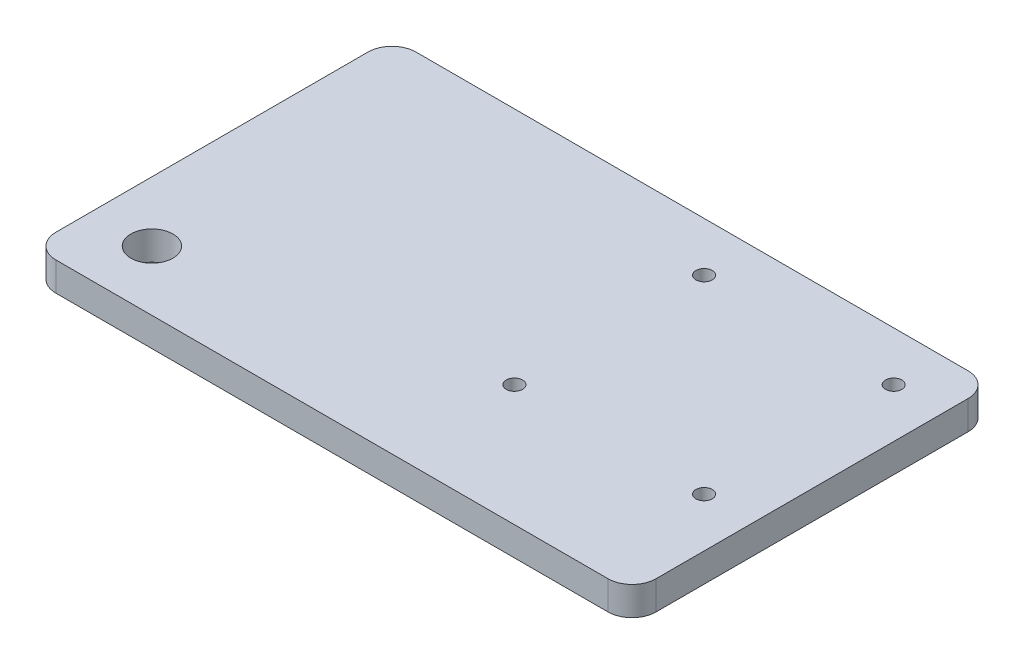
SolidWorks part; units mm, degrees
material "A3钢"
ref_plane "前视基准面" through (0, 0, 0) normal (0, 0, 1) x (1, 0, 0)
ref_plane "上视基准面" through (0, 0, 0) normal (0, 1, 0) x (1, 0, 0)
ref_plane "右视基准面" through (0, 0, 0) normal (1, 0, 0) x (0, 0, -1)
sketch "草图1" plane through (0, 0, 0) normal (0, 1, 0) x (1, 0, 0)
  line L1 (-125, 75) -> (125, 75)
  line L2 (-125, 75) -> (-125, -75)
  line L3 (-125, -75) -> (125, -75)
  line L4 (125, 75) -> (125, -75)
  line L5 (-125, 75) -> (125, -75) construction
  line L6 (-125, -75) -> (125, 75) construction
  point P0 (0, 0)
  dimension "D1" = 150
  dimension "D2" = 250
extrude "凸台-拉伸1" add sketch "草图1" along normal blind 12
hole_wizard "M20 螺纹孔1" positions "草图2" profile "草图3" tap size "M20" standard "GB" end condition through all
sketch "草图2" plane through (0, 0, 0) normal (0, -1, 0) x (-1, 0, 0)
  line L0 (125, 75) -> (125, -75) construction
  line L1 (125, -75) -> (-125, -75) construction
  point P0 (100, -50)
  dimension "D1" = 25
  dimension "D2" = 25
cosmetic thread "孔螺蚊线1" parameters "D2"=20
sketch "草图3" plane through (-100, 0, 50) normal (1, 0, 0) x (0, 0, -1)
  line L0 (0, 0) -> (0, 12)
  line L1 (0, 12) -> (8.75, 12)
  line L2 (8.75, 12) -> (8.75, 0)
  line L5 (8.75, 0) -> (0, 0)
  line L11 (0, -6.35) -> (0, 107.95) construction
  dimension "通孔螺纹孔钻头直径" = 17.5
  dimension "通孔螺纹孔钻头深度" = 12
hole_wizard "M8 螺纹孔1" positions "草图4" profile "草图5" tap size "M8" standard "GB" end condition through all
sketch "草图4" plane through (0, 12, 0) normal (0, 1, 0) x (1, 0, 0)
  line L0 (25.5, 54.5) -> (104.5, 54.5) construction
  line L1 (104.5, 54.5) -> (104.5, -24.5) construction
  line L2 (104.5, -24.5) -> (25.5, -24.5) construction
  line L3 (25.5, -24.5) -> (25.5, 54.5) construction
  line L9 (65, 54.5) -> (65, -24.5) construction
  line L12 (125, -75) -> (125, 75) construction
  line L13 (25.5, 15) -> (104.5, 15) construction
  line L17 (125, 75) -> (-125, 75) construction
  point P0 (25.5, 54.5)
  point P2 (104.5, 54.5)
  point P4 (25.5, -24.5)
  point P6 (104.5, -24.5)
  dimension "D1" = 60
  dimension "D2" = 79
  dimension "D3" = 79
  dimension "D4" = 60
sketch "草图5" plane through (25.5, 12, -54.5) normal (1, 0, 0) x (0, 0, 1)
  line L0 (0, 0) -> (0, 12)
  line L1 (0, 12) -> (3.4, 12)
  line L2 (3.4, 12) -> (3.4, 0)
  line L5 (3.4, 0) -> (0, 0)
  line L11 (0, -6.35) -> (0, 107.95) construction
  dimension "通孔螺纹孔钻头直径" = 6.8
  dimension "通孔螺纹孔钻头深度" = 12
cosmetic thread "孔螺蚊线2" parameters "D2"=8
cosmetic thread "孔螺蚊线3" parameters "D2"=8
cosmetic thread "孔螺蚊线4" parameters "D2"=8
cosmetic thread "孔螺蚊线5" parameters "D2"=8
fillet "圆角1" radius 10 4 edges at (-125, 6, -75) (125, 6, -75) (125, 6, 75) (-125, 6, 75)
hole_wizard "Ø5.5 (5.5) 直径孔1" positions "草图6" profile "草图7" hole size "Ø5.5" standard "GB"
sketch "草图6" [suppressed] plane through (0, 0, 0) normal (0, -1, 0) x (-1, 0, 0)
  line L0 (-35.5, -14.5) -> (-114.5, 64.5) construction
  point P0 (-75, 25)
sketch "草图7" plane through (75, 0, -25) normal (1, 0, 0) x (0, 0, -1)
  line L0 (0, 0) -> (0, 12)
  line L1 (0, 12) -> (2.75, 12)
  line L2 (2.75, 12) -> (2.75, 0)
  line L5 (2.75, 0) -> (0, 0)
  line L11 (0, -6.35) -> (0, 107.95) construction
  dimension "通孔孔直径" = 5.5
  dimension "通孔孔深度" = 12
sketch "草图8" plane through (0, 0, 0) normal (0, -1, 0) x (1, 0, 0)
  circle A0 centre (-100, 50) radius 10.5
  dimension "D1" = 21
extrude "切除-拉伸1" [suppressed] cut sketch "草图8" against normal blind 64
sketch "草图9" [suppressed] plane through (0, 0, 0) normal (0, -1, 0) x (1, 0, 0)
  line L1 (-92.6795, 50) -> (-101.3397, 65)
  line L2 (-101.3397, 65) -> (-118.6603, 65)
  line L3 (-118.6603, 65) -> (-127.3205, 50)
  line L4 (-127.3205, 50) -> (-118.6603, 35)
  line L5 (-118.6603, 35) -> (-101.3397, 35)
  line L6 (-101.3397, 35) -> (-92.6795, 50)
  circle A0 centre (-110, 50) radius 15 construction
  circle A1 centre (-110, 50) radius 5
  dimension "D1" = 10
  dimension "D2" = 30
extrude "凸台-拉伸2" [suppressed] add sketch "草图9" along normal blind 16
hole_wizard "M20 螺纹孔2" positions "草图10" profile "草图11" tap size "M20" standard "GB"
sketch "草图10" [suppressed] plane through (0, -16, 0) normal (0, -1, 0) x (-1, 0, 0)
  point P0 (110, -50)
sketch "草图11" plane through (-110, -16, 50) normal (1, 0, 0) x (0, 0, -1)
  line L0 (0, 0) -> (0, 28)
  line L1 (0, 28) -> (8.75, 28)
  line L2 (8.75, 28) -> (8.75, 0)
  line L5 (8.75, 0) -> (0, 0)
  line L11 (0, -6.35) -> (0, 107.95) construction
  dimension "通孔螺纹孔钻头直径" = 17.5
  dimension "通孔螺纹孔钻头深度" = 28
cosmetic thread "孔螺蚊线6" [suppressed] parameters "D1"=0, "D2"=18.5
